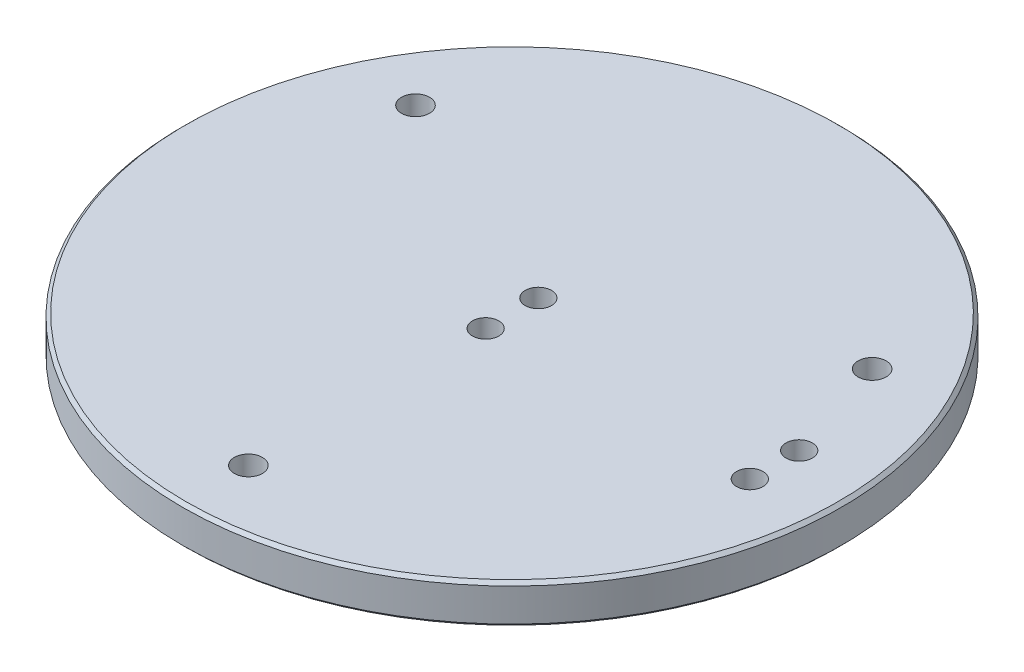
from build123d import *

# Parameters (mm, degrees)
SKETCH2_R                               = 100
BOSS_EXTRUDE1_DEPTH                     = 12
M10_TAPPED_HOLE1_D                      = 8.5
M10_TAPPED_HOLE1_DEPTH                  = 24.5
M10_TAPPED_HOLE1_TIP                    = 2.553657631
CBORE_FOR_M4_HEX_HEAD_BOLT1_D           = 4.5
CBORE_FOR_M4_HEX_HEAD_BOLT1_DEPTH       = 24.5
CBORE_FOR_M4_HEX_HEAD_BOLT1_CBORE_D     = 8
CBORE_FOR_M4_HEX_HEAD_BOLT1_CBORE_DEPTH = 7
CBORE_FOR_M4_HEX_HEAD_BOLT1_TIP         = 1.351936393
CHAMFER1_SIZE                           = 1


with BuildPart() as part:
    # Sketch2 → Boss-Extrude1 (new body)
    with BuildSketch(Plane(origin=(0, 0, 0), x_dir=(1, 0, 0), z_dir=(0, 1, 0))):
        with Locations(Location((0, 0, 0), (0, 0, 270))):
            Circle(SKETCH2_R)
    extrude(amount=-BOSS_EXTRUDE1_DEPTH)

    # M10 Tapped Hole1
    with Locations(Plane(origin=(-69.282032303, 0, -40), x_dir=(0, 0, 1), z_dir=(0, 1, 0))):
        with Locations((0, 0), (0, 138.564064606), (120, 69.282032303)):
            Hole(M10_TAPPED_HOLE1_D / 2, depth=M10_TAPPED_HOLE1_DEPTH)
            with Locations((0, 0, -(M10_TAPPED_HOLE1_DEPTH + M10_TAPPED_HOLE1_TIP / 2))):  # 118° drill point
                Cone(0, M10_TAPPED_HOLE1_D / 2, M10_TAPPED_HOLE1_TIP, mode=Mode.SUBTRACT)

    # CBORE for M4 Hex Head Bolt1
    with Locations(Plane(origin=(79.64766161, 0, -7.5), x_dir=(0, 0, 1), z_dir=(0, 1, 0))):
        with Locations((0, 0), (15, 0), (15.5, -79.64766161), (-0.5, -79.64766161)):
            CounterBoreHole(CBORE_FOR_M4_HEX_HEAD_BOLT1_D / 2, CBORE_FOR_M4_HEX_HEAD_BOLT1_CBORE_D / 2, CBORE_FOR_M4_HEX_HEAD_BOLT1_CBORE_DEPTH, depth=CBORE_FOR_M4_HEX_HEAD_BOLT1_DEPTH)
            with Locations((0, 0, -(CBORE_FOR_M4_HEX_HEAD_BOLT1_DEPTH + CBORE_FOR_M4_HEX_HEAD_BOLT1_TIP / 2))):  # 118° drill point
                Cone(0, CBORE_FOR_M4_HEX_HEAD_BOLT1_D / 2, CBORE_FOR_M4_HEX_HEAD_BOLT1_TIP, mode=Mode.SUBTRACT)

    # Chamfer1
    chamfer1_edges = [part.edges().sort_by_distance(p)[0] for p in [
        (0, 0, -100),
        (0, -12, -100),
    ]]
    chamfer(chamfer1_edges, length=CHAMFER1_SIZE)


solid = part.part
